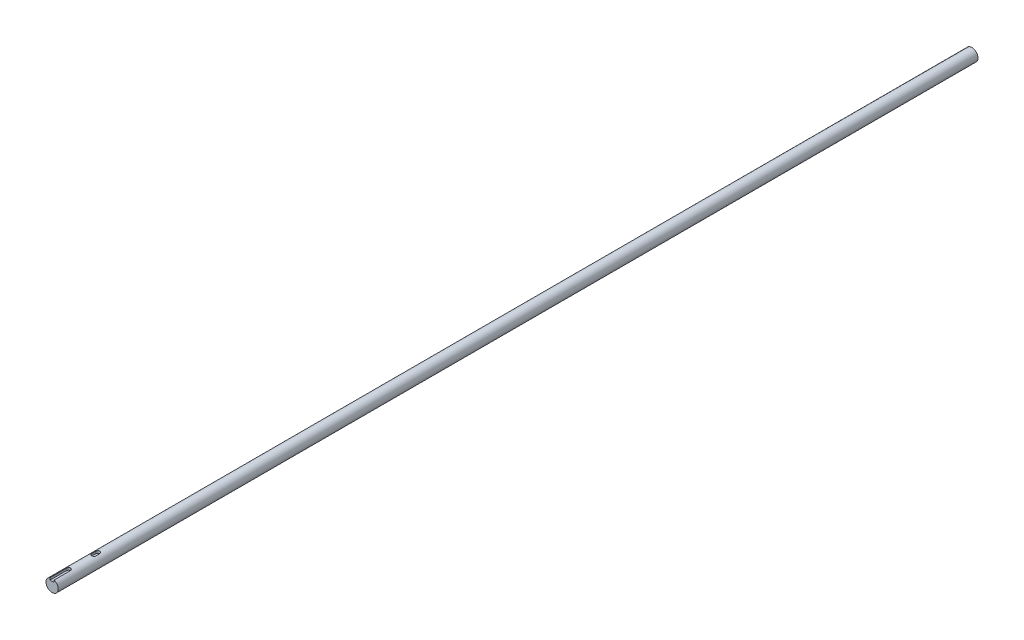
from build123d import *

# Parameters (mm, degrees)
SKETCH_1_R               = 7.5
EXTRUDE_1_DEPTH          = 1130
CUT_EXTRUDE_START        = -20
CUT_EXTRUDE_1_DEPTH      = 20
CUT_EXTRUDE_2_REACH      = 1132.089
CUT_EXTRUDE_2_END_RADIUS = 7.5
CUT_EXTRUDE_3_DEPTH      = 17


with BuildPart() as part:
    # 草图1 → 凸台-拉伸1 (new body)
    with BuildSketch(Plane.XY):
        Circle(SKETCH_1_R)
    extrude(amount=EXTRUDE_1_DEPTH)

    # 草图2 → 切除-拉伸1 (cut)
    with BuildSketch(Plane.XY.offset(1130).offset(CUT_EXTRUDE_START)):
        with BuildLine():
            Line((-2.5, 7.071067812), (-2.5, 4.5))
            Line((-2.5, 4.5), (2.5, 4.5))
            Line((2.5, 4.5), (2.5, 7.071067812))
            ThreePointArc((2.5, 7.071067812), (0, 7.5), (-2.5, 7.071067812))
        make_face()
    extrude(amount=CUT_EXTRUDE_1_DEPTH, mode=Mode.SUBTRACT)

    # 切除-拉伸2: up to this cylinder (the profile starts inside it)
    cut_extrude_2_end = Plane(origin=(0, 0, 1108.938967), z_dir=(0, 0, -1)) * Cylinder(CUT_EXTRUDE_2_END_RADIUS, 2280.178, mode=Mode.PRIVATE)
    # 草图3 → 切除-拉伸2 (cut, up to the surface)
    with BuildSketch(Plane(origin=(0, 4.5, 0), x_dir=(1, 0, 0), z_dir=(0, 1, 0)), mode=Mode.PRIVATE) as cut_extrude_2_sk1:
        with BuildLine():
            Line((-2.5, -1110), (2.5, -1110))
            ThreePointArc((2.5, -1110), (0, -1107.5), (-2.5, -1110))
        make_face()
    cut_extrude_2_tool1 = extrude(cut_extrude_2_sk1.sketch, amount=CUT_EXTRUDE_2_REACH, mode=Mode.PRIVATE) & cut_extrude_2_end
    add(cut_extrude_2_tool1.solids().sort_by_distance((0, 4.5, 1108.938967))[0], mode=Mode.SUBTRACT)

    # 草图5 → 切除-拉伸3 (cut)
    with BuildSketch(Plane(origin=(0, 4.5, 0), x_dir=(1, 0, 0), z_dir=(0, 1, 0))):
        with BuildLine():
            Line((-2.5, -1079.079030824), (-2.5, -1074.079030824))
            ThreePointArc((-2.5, -1074.079030824), (0, -1071.579030824), (2.5, -1074.079030824))
            Line((2.5, -1074.079030824), (2.5, -1079.079030824))
            ThreePointArc((2.5, -1079.079030824), (0, -1081.579030824), (-2.5, -1079.079030824))
        make_face()
    extrude(amount=CUT_EXTRUDE_3_DEPTH, mode=Mode.SUBTRACT)


solid = part.part
